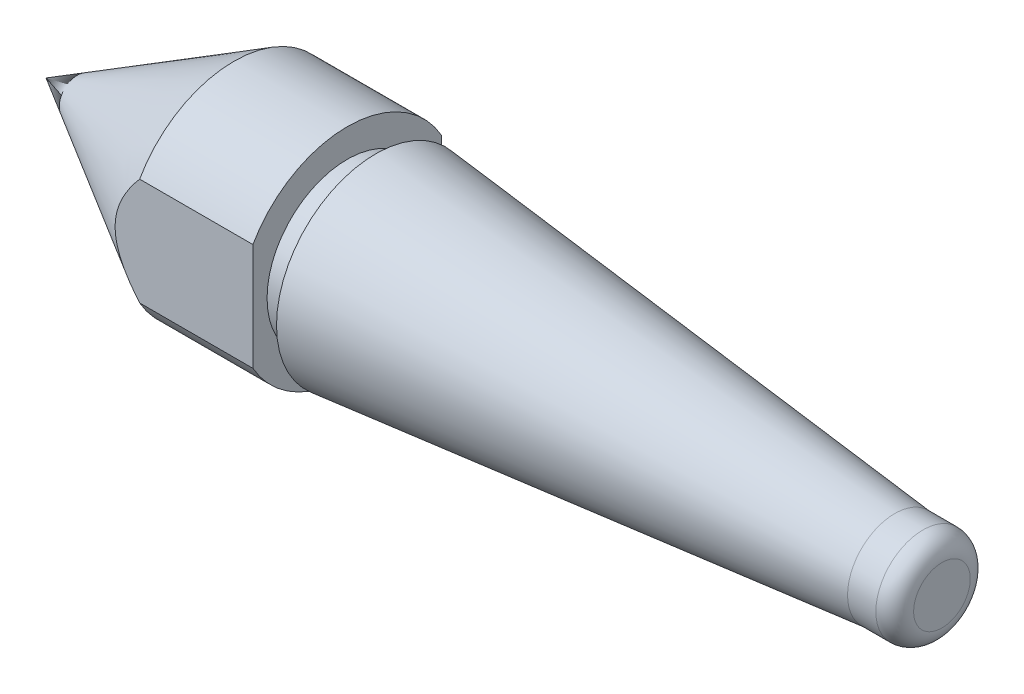
from build123d import *

# Parameters (mm, degrees)
FILLET1_R          = 2
CUT_EXTRUDE1_DEPTH = 66.065351763


with BuildPart() as part:
    # Sketch1 → Revolve1 (revolve)
    with BuildSketch(Plane.XY, mode=Mode.PRIVATE) as revolve1_sk:
        Polygon((0, 0), (0, 5), (-5, 5), (-60, 10.5), (-60, 8.5), (-63, 8.5), (-63, 11.5), (-75, 11.5), (-94.92, 0), align=None)
    revolve(revolve1_sk.sketch.rotate(Axis((-94.92, 0, 0), (1, 0, 0)), 90), axis=Axis((-94.92, 0, 0), (1, 0, 0)))

    # Fillet1
    fillet1_edges = [part.edges().sort_by_distance(p)[0] for p in [
        (0, 0, -5),
    ]]
    fillet(fillet1_edges, radius=FILLET1_R)

    # Sketch2 → Cut-Extrude1 (cut, through all)
    with BuildSketch(Plane(origin=(-63, 0, 0), x_dir=(0, 0, -1), z_dir=(1, 0, 0))):
        with BuildLine():
            Line((-10, 5.678908346), (-10, -5.678908346))
            ThreePointArc((-10, -5.678908346), (-11.5, 0), (-10, 5.678908346))
        make_face()
        with BuildLine():
            Line((10, 5.678908346), (10, -5.678908346))
            ThreePointArc((10, -5.678908346), (11.5, 0), (10, 5.678908346))
        make_face()
    extrude(amount=-CUT_EXTRUDE1_DEPTH, mode=Mode.SUBTRACT)


solid = part.part
